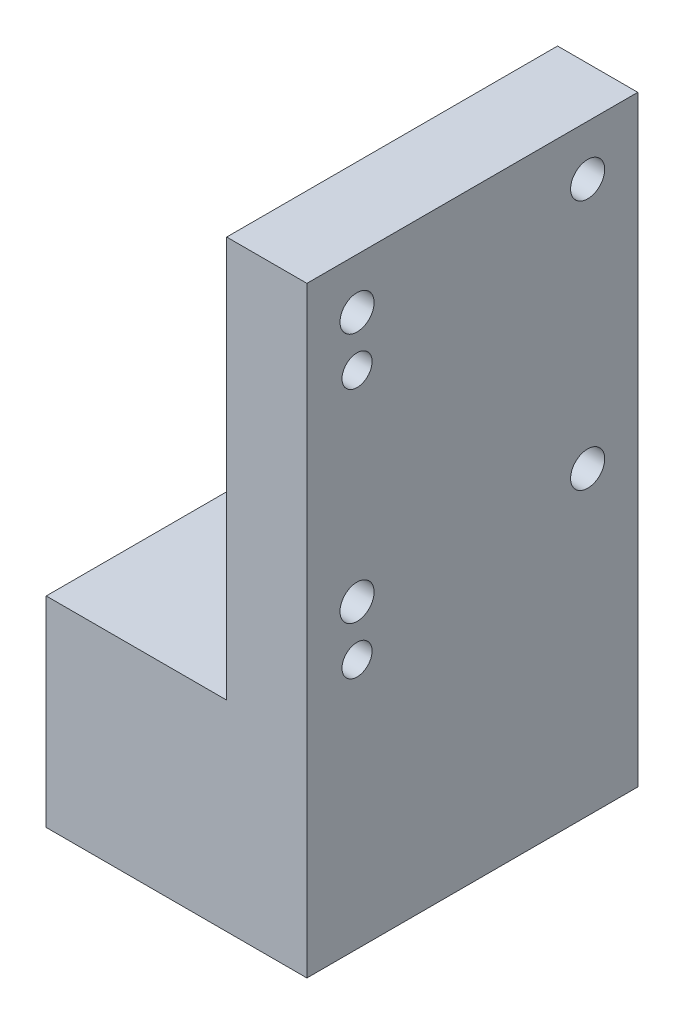
SolidWorks part; units mm, degrees
ref_plane "Front Plane" through (0, 0, 0) normal (0, 0, 1) x (1, 0, 0)
ref_plane "Top Plane" through (0, 0, 0) normal (0, 1, 0) x (1, 0, 0)
ref_plane "Right Plane" through (0, 0, 0) normal (1, 0, 0) x (0, 0, -1)
sketch "Sketch 1" plane through (0, 0, 0) normal (1, 0, 0) x (0, 0, -1)
  line L1 (-16.5, -30) -> (16.5, -30)
  line L2 (-16.5, -30) -> (-16.5, 30)
  line L3 (-16.5, 30) -> (16.5, 30)
  line L4 (16.5, -30) -> (16.5, 30)
  line L5 (-16.5, -30) -> (16.5, 30) construction
  line L6 (-16.5, 30) -> (16.5, -30) construction
  point P0 (0, 0)
  dimension "D1" = 60
  dimension "D2" = 33
extrude "Boss-Extrude 1" add sketch "Sketch 1" along normal blind 8
sketch "Sketch 2" plane through (0, 0, 0) normal (-1, 0, 0) x (0, 0, 1)
  line L0 (16.5, 30) -> (16.5, -30) construction
  line L1 (-16.5, -30) -> (16.5, -30)
  line L2 (-16.5, -30) -> (-16.5, -5)
  line L3 (-16.5, -5) -> (16.5, -5)
  line L4 (16.5, -30) -> (16.5, -5)
  dimension "D1" = 25
extrude "Boss-Extrude 2" add sketch "Sketch 2" along normal blind 18
hole_wizard "M3 Hex Socket Cap Screw Counterbore 1" positions "Sketch 4" profile "Sketch 3" counterbore size "M3" standard "ISO" end condition through all
sketch "Sketch 4" plane through (0, 0, 0) normal (-1, 0, 0) x (0, 0, 1)
  line L0 (-16.5, 30) -> (16.5, 30) construction
  point P0 (-11.5, 25)
  dimension "D1" = 11.5
  dimension "D2" = 5
sketch "Sketch 3" plane through (0, 25, -11.5) normal (0, 1, 0) x (0, 0, 1)
  line L0 (0, 0) -> (0, 8)
  line L1 (0, 8) -> (1.7, 8)
  line L3 (1.7, 8) -> (1.7, 3)
  line L4 (1.7, 3) -> (3.25, 3)
  line L5 (3.25, 3) -> (3.25, 0)
  line L7 (3.25, 0) -> (0, 0)
  line L11 (0, -6.35) -> (0, 107.95) construction
  dimension "貫穿孔直徑" = 3.4
  dimension "貫穿孔深度" = 8
  dimension "柱孔直徑" = 6.5
  dimension "柱孔深度" = 3
pattern_linear "Linear Pattern 1" count 2 spacing 23 along (0, 0, 1) count 2 spacing 25 along (0, -1, 0) of "M3 Hex Socket Cap Screw Counterbore 1"
hole_wizard "M4 Tapped Hole 2" positions "Sketch 8" profile "Sketch 7" tap size "M4" standard "GB"
sketch "Sketch 8" plane through (-18, 0, 0) normal (-1, 0, 0) x (0, 0, 1)
  line L0 (-16.5, -30) -> (16.5, -30) construction
  line L1 (-16.5, -5) -> (-16.5, -30) construction
  point P0 (0, -25)
  dimension "D1" = 5
  dimension "D2" = 16.5
sketch "Sketch 7" plane through (-18, -25, 0) normal (0, 1, 0) x (0, 0, 1)
  line L0 (0, 0) -> (0, 11.0914)
  line L1 (0, 11.0914) -> (1.65, 10.1)
  line L2 (1.65, 10.1) -> (1.65, 0)
  line L5 (1.65, 0) -> (0, 0)
  line L10 (0, 11.0914) -> (-1.65, 10.1) construction
  line L11 (0, -6.35) -> (0, 107.95) construction
  dimension "螺孔鑽直徑" = 3.3
  dimension "螺孔鑽深度" = 10.1
  dimension "導頭角度" = 118
cosmetic thread "Cosmetic Thread 2" parameters "D1"=8, "D2"=4
pattern_linear "Linear Pattern 2" count 2 spacing 10 along (0, 1, 0) of "M4 Tapped Hole 2"
sketch "Sketch 9" plane through (-18, 0, 0) normal (-1, 0, 0) x (0, 0, 1)
  line L0 (16.5, -30) -> (16.5, -5) construction
  line L1 (-16.5, -5) -> (16.5, -5)
  line L2 (-16.5, -5) -> (-16.5, -10)
  line L3 (-16.5, -10) -> (16.5, -10)
  line L4 (16.5, -5) -> (16.5, -10)
  dimension "D1" = 5
extrude "Cut-Extrude 1" cut sketch "Sketch 9" against normal up to surface (18 mm away) up to face at (0, 25, 14.75)
hole_wizard "Ø3.0 (3) Hole 1" positions "Sketch 11" profile "Sketch 10" hole size "Ø3.0" standard "GB" end condition through all
sketch "Sketch 11" plane through (0, 0, 0) normal (-1, 0, 0) x (0, 0, 1)
  line L0 (16.5, 30) -> (16.5, -10) construction
  circle A0 centre (11.5, 25) radius 1.7 construction
  point P0 (11.5, 20)
  dimension "D2" = 5
  dimension "D1" = 5
sketch "Sketch 10" plane through (0, 20, 11.5) normal (0, 1, 0) x (0, 0, 1)
  line L0 (0, 0) -> (0, 8)
  line L1 (0, 8) -> (1.5, 8)
  line L2 (1.5, 8) -> (1.5, 0)
  line L5 (1.5, 0) -> (0, 0)
  line L11 (0, -6.35) -> (0, 107.95) construction
  dimension "貫穿孔直徑" = 3
  dimension "貫穿孔深度" = 8
pattern_linear "Linear Pattern 3" count 2 spacing 25 along (0, -1, 0) of "Ø3.0 (3) Hole 1"
hole_wizard "Ø4.0 (4) Hole 1" positions "Sketch 13" profile "Sketch 12" hole size "Ø4.0" standard "JIS"
sketch "Sketch 13" plane through (-18, 0, 0) normal (-1, 0, 0) x (0, 0, 1)
  line L0 (-16.5, -30) -> (16.5, -30) construction
  point P0 (-8, -20)
  point P3 (0, -30)
  dimension "D1" = 8
  dimension "D2" = 10
sketch "Sketch 12" plane through (-18, -20, -8) normal (0, 1, 0) x (0, 0, 1)
  line L0 (0, 0) -> (0, 11.2017)
  line L1 (0, 11.2017) -> (2, 10)
  line L2 (2, 10) -> (2, 0)
  line L5 (2, 0) -> (0, 0)
  line L10 (0, 11.2017) -> (-2, 10) construction
  line L11 (0, -6.35) -> (0, 107.95) construction
  dimension "鑽孔直徑" = 4
  dimension "鑽孔深度" = 10
  dimension "導頭角度" = 118
pattern_linear "Linear Pattern 4" count 2 spacing 16 along (0, 0, 1) of "Ø4.0 (4) Hole 1"
